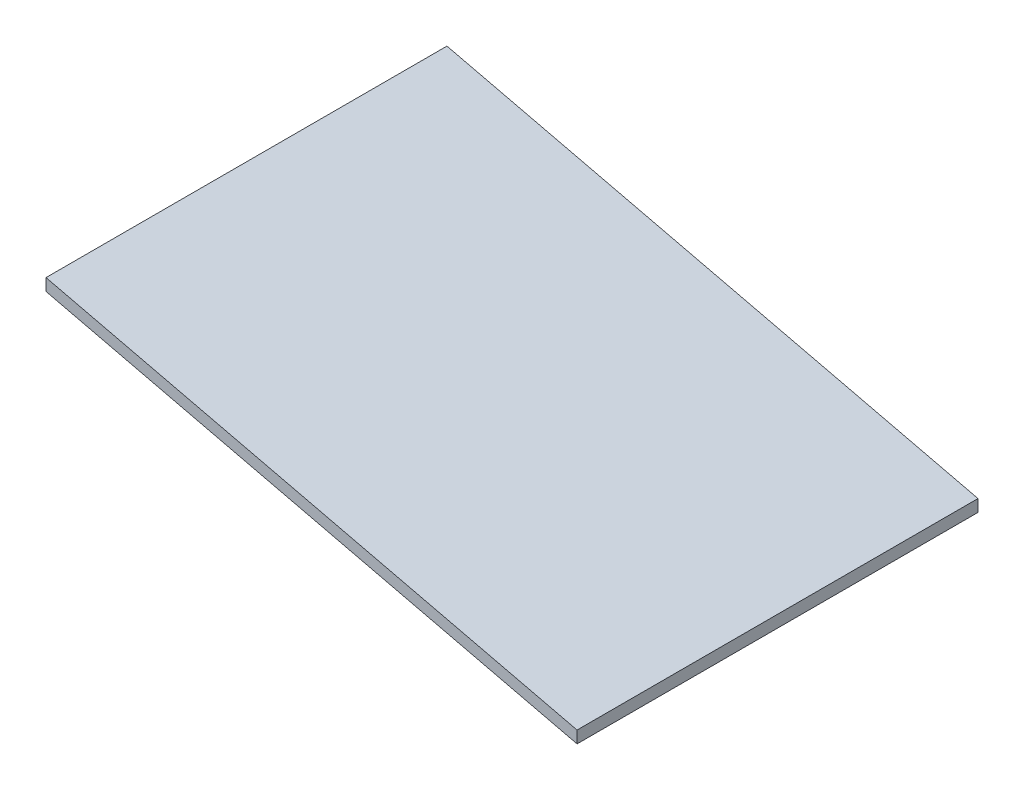
from build123d import *

# Parameters (mm, degrees)
EXTRUDE_1_DEPTH = 1000


with BuildPart() as part:
    # 草图1 → 凸台-拉伸1 (new body)
    with BuildSketch(Plane.XY):
        Polygon((0, 0), (1324.500000007, -314.999999957), (1324.500000007, -344.999999957), (0, -30), align=None)
    extrude(amount=EXTRUDE_1_DEPTH)


solid = part.part
